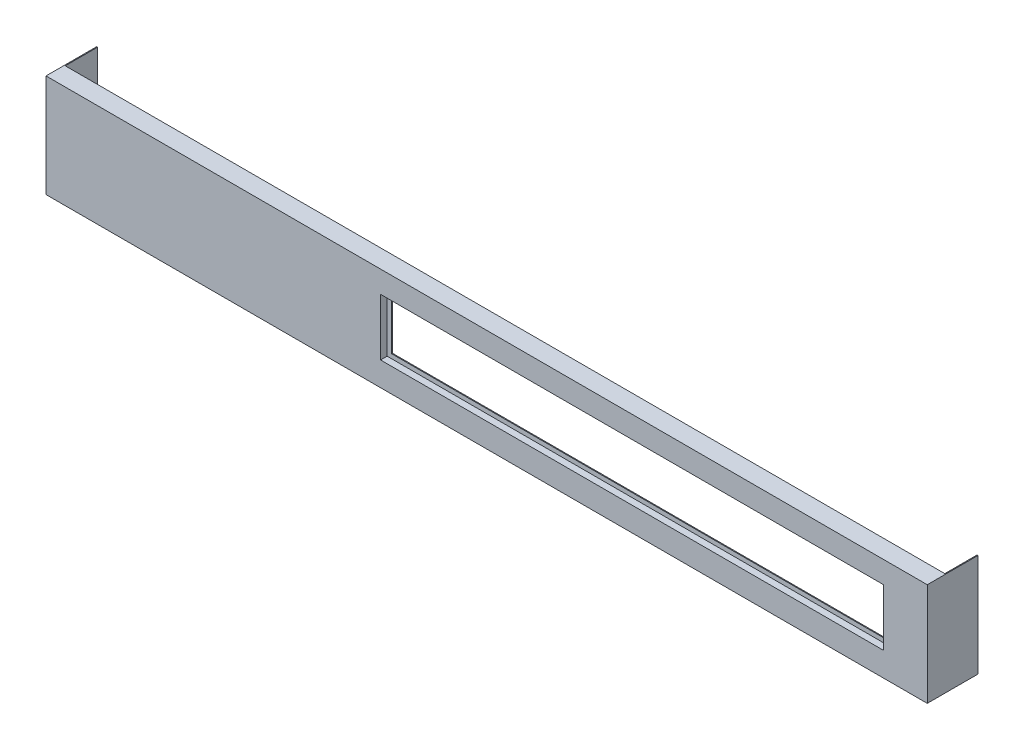
from build123d import *

# Parameters (mm, degrees)
SKETCH_2_W          = 2015
SKETCH_2_H          = 235
EXTRUDE_1_DEPTH     = 2
SKETCH_3_W          = 2
SKETCH_3_H          = 235
EXTRUDE_2_DEPTH     = 114
SKETCH_4_W          = 2011
SKETCH_4_H          = 2
EXTRUDE_3_DEPTH     = 40
SKETCH_5_W          = 1150
SKETCH_5_H          = 130
CUT_EXTRUDE_1_DEPTH = 10
SKETCH_6_W          = 2015
SKETCH_6_H          = 42
EXTRUDE_4_DEPTH     = 2
SKETCH_7_W          = 1154
SKETCH_7_H          = 134
SKETCH_7_W_2        = 1150
SKETCH_7_H_2        = 130
EXTRUDE_5_DEPTH     = 15
SKETCH_8_W          = 1154
SKETCH_8_H          = 134
SKETCH_8_W_2        = 1130
SKETCH_8_H_2        = 110
EXTRUDE_6_DEPTH     = 2


with BuildPart() as part:
    # 草图2 → 凸台-拉伸1 (new body)
    with BuildSketch(Plane.XY):
        with Locations((1007.5, 117.5)):
            Rectangle(SKETCH_2_W, SKETCH_2_H)
    extrude(amount=EXTRUDE_1_DEPTH)

    # 草图3 → 凸台-拉伸2 (add)
    with BuildSketch(Plane(origin=(0, 0, 0), x_dir=(-1, 0, 0), z_dir=(0, 0, -1))):
        with Locations((-2014, 117.5)):
            Rectangle(SKETCH_3_W, SKETCH_3_H)
        with Locations((-1, 117.5)):
            Rectangle(SKETCH_3_W, SKETCH_3_H)
    extrude(amount=EXTRUDE_2_DEPTH)

    # 草图4 → 凸台-拉伸3 (add)
    with BuildSketch(Plane(origin=(0, 0, 0), x_dir=(-1, 0, 0), z_dir=(0, 0, -1))):
        with Locations((-1007.5, 234)):
            Rectangle(SKETCH_4_W, SKETCH_4_H)
    extrude(amount=EXTRUDE_3_DEPTH)

    # 草图5 → 切除-拉伸1 (cut)
    with BuildSketch(Plane.XY.offset(2)):
        with Locations((1340, 120)):
            Rectangle(SKETCH_5_W, SKETCH_5_H)
    extrude(amount=-CUT_EXTRUDE_1_DEPTH, mode=Mode.SUBTRACT)

    # 草图6 → 凸台-拉伸4 (add)
    with BuildSketch(Plane.XZ):
        with Locations((1007.5, -19)):
            Rectangle(SKETCH_6_W, SKETCH_6_H)
    extrude(amount=-EXTRUDE_4_DEPTH)

    # 草图7 → 凸台-拉伸5 (add)
    with BuildSketch(Plane(origin=(0, 0, 0), x_dir=(-1, 0, 0), z_dir=(0, 0, -1))):
        with Locations((-1340, 120)):
            Rectangle(SKETCH_7_W, SKETCH_7_H)
        with Locations((-1340, 120)):
            Rectangle(SKETCH_7_W_2, SKETCH_7_H_2, mode=Mode.SUBTRACT)
    extrude(amount=EXTRUDE_5_DEPTH)

    # 草图8 → 凸台-拉伸6 (add)
    with BuildSketch(Plane(origin=(0, 0, -15), x_dir=(-1, 0, 0), z_dir=(0, 0, -1))):
        with Locations((-1340, 120)):
            Rectangle(SKETCH_8_W, SKETCH_8_H)
        with Locations((-1340, 120)):
            Rectangle(SKETCH_8_W_2, SKETCH_8_H_2, mode=Mode.SUBTRACT)
    extrude(amount=-EXTRUDE_6_DEPTH)


solid = part.part
